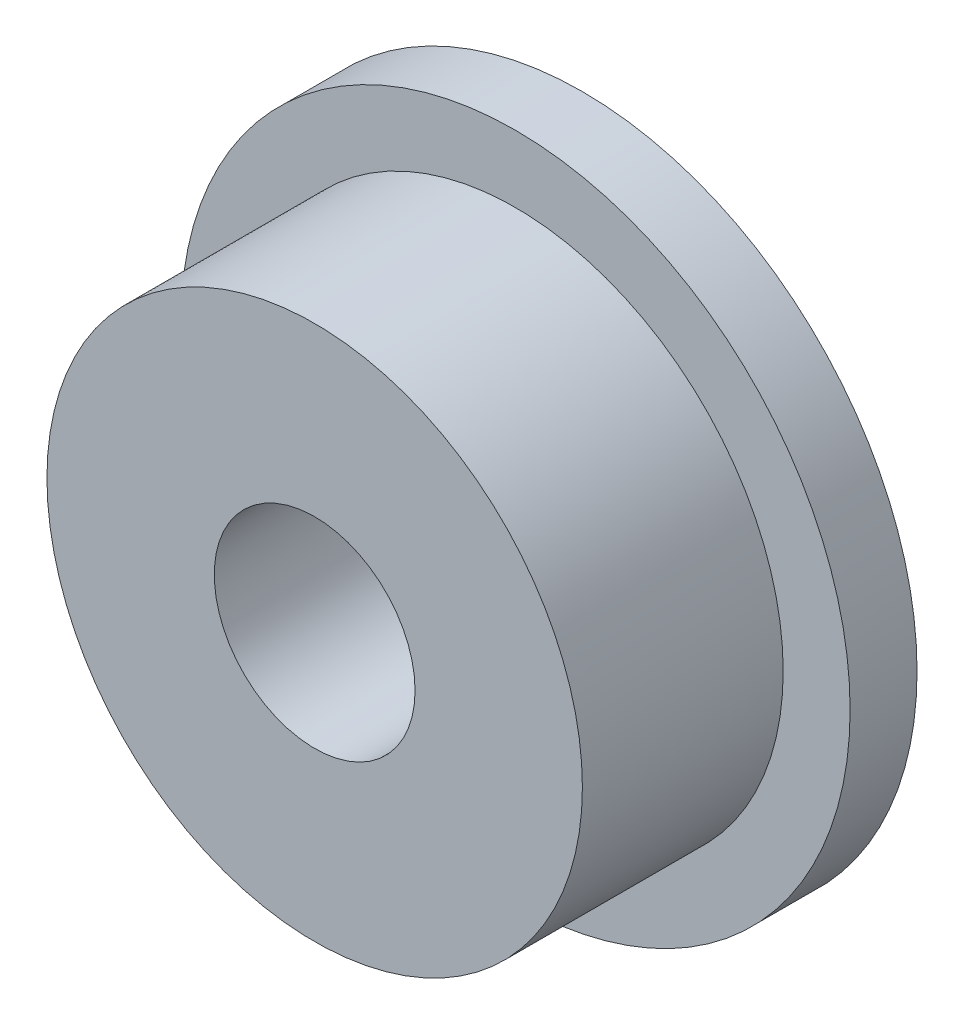
from build123d import *

# Parameters (mm, degrees)
SKETCH1_R               = 5
BOSS_EXTRUDE1_DEPTH     = 4
CUT_EXTRUDE1_START      = -3
SKETCH2_R               = 5
SKETCH2_R_2             = 4
CUT_EXTRUDE1_DEPTH      = 3
CUT_EXTRUDE2_DEPTH      = 9.124038405
CUT_EXTRUDE2_DEPTH_BACK = 9.124038405
SKETCH3_R               = 1.5


with BuildPart() as part:
    # Sketch1 → Boss-Extrude1 (new body)
    with BuildSketch(Plane.XY):
        Circle(SKETCH1_R)
    extrude(amount=BOSS_EXTRUDE1_DEPTH)

    # Sketch2 → Cut-Extrude1 (cut)
    with BuildSketch(Plane.XY.offset(4).offset(CUT_EXTRUDE1_START)):
        Circle(SKETCH2_R)
        Circle(SKETCH2_R_2, mode=Mode.SUBTRACT)
    extrude(amount=CUT_EXTRUDE1_DEPTH, mode=Mode.SUBTRACT)

    # Sketch3 → Cut-Extrude2 (cut, two sides: drawn at the far end of the back side and taken through both)
    with BuildSketch(Plane.XY.offset(4).offset(-CUT_EXTRUDE2_DEPTH_BACK)):
        Circle(SKETCH3_R)
    extrude(amount=CUT_EXTRUDE2_DEPTH + CUT_EXTRUDE2_DEPTH_BACK, mode=Mode.SUBTRACT)


solid = part.part
